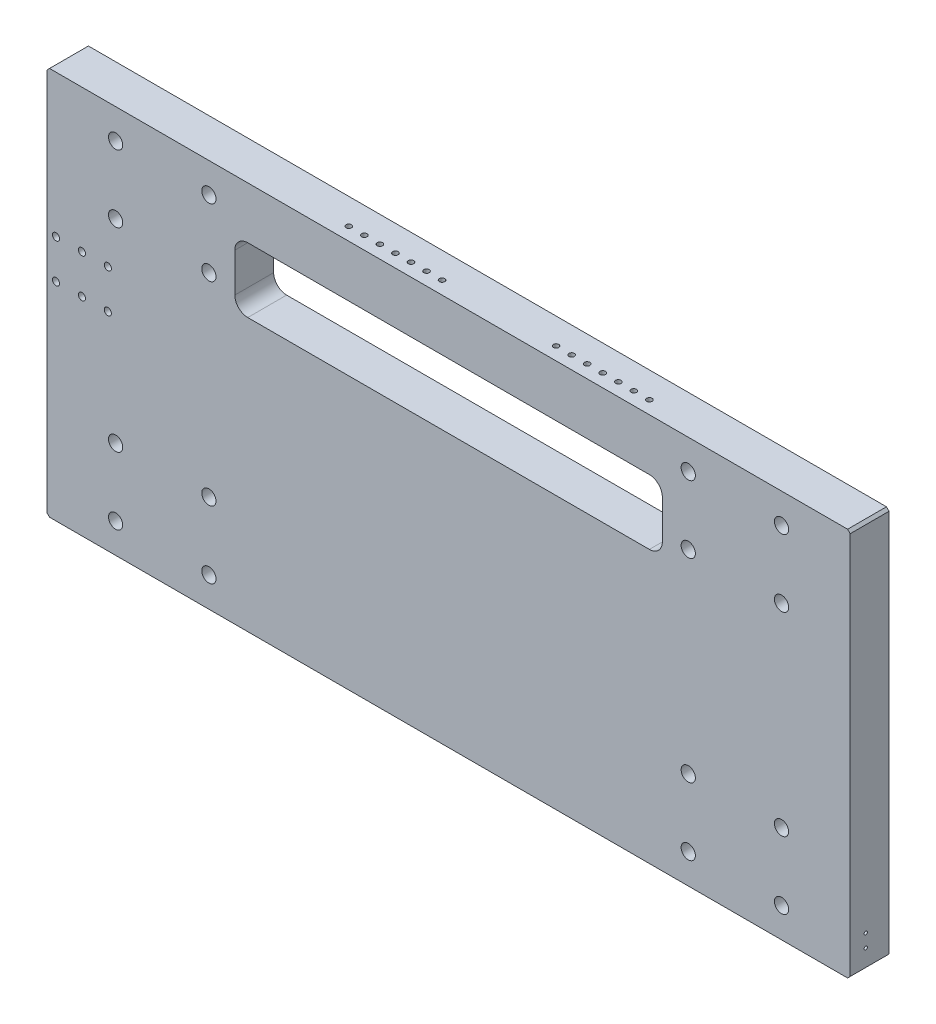
from build123d import *

# Parameters (mm, degrees)
SKETCH1_W                                            = 620
SKETCH1_H                                            = 300
BOSS_EXTRUDE1_DEPTH                                  = 15
CUT_EXTRUDE2_DEPTH                                   = 346.687720349
CHAMFER1_SIZE                                        = 2
M12_TAPPED_HOLE1_AT_2_COUNT                          = 2
M12_TAPPED_HOLE1_AT_2_PITCH                          = 190
M12_TAPPED_HOLE1_AT_3_COUNT                          = 2
M12_TAPPED_HOLE1_AT_3_PITCH                          = 447.353327919
M12_TAPPED_HOLE1_AT_4_COUNT                          = 2
M12_TAPPED_HOLE1_AT_4_PITCH                          = 405
LPATTERN1_COUNT                                      = 2
LPATTERN1_PITCH                                      = 35
M5_TAPPED_HOLE1_D                                    = 4.2
M5_TAPPED_HOLE1_DEPTH                                = 12.4
M5_TAPPED_HOLE1_TIP                                  = 1.2618073
F_4_0_4_DIAMETER_HOLE1_D                             = 4
F_4_0_4_DIAMETER_HOLE1_DEPTH                         = 12
F_4_0_4_DIAMETER_HOLE1_TIP                           = 1.201721238
HOLE_SIZE_PER_SOCKET_HEAD_CAP_SCREW_TYPE_D           = 11
HOLE_SIZE_PER_SOCKET_HEAD_CAP_SCREW_TYPE_CBORE_D     = 18
HOLE_SIZE_PER_SOCKET_HEAD_CAP_SCREW_TYPE_CBORE_DEPTH = 11
HOLE_SIZE_PER_SOCKET_HEAD_CAP_SCREW_2_D              = 5.5
HOLE_SIZE_PER_SOCKET_HEAD_CAP_SCREW_2_CBORE_D        = 10
HOLE_SIZE_PER_SOCKET_HEAD_CAP_SCREW_2_CBORE_DEPTH    = 5.7
M3_TAPPED_HOLE2_AT_2_COUNT                           = 2
M3_TAPPED_HOLE2_AT_2_PITCH                           = 10
M5_TAPPED_HOLE2_D                                    = 4.2
M5_TAPPED_HOLE2_DEPTH                                = 14
M5_TAPPED_HOLE2_TIP                                  = 1.2618073
M8_TAPPED_HOLE1_D                                    = 6.8
M8_TAPPED_HOLE1_DEPTH                                = 26.25
M8_TAPPED_HOLE1_TIP                                  = 2.042926105
M5_TAPPED_HOLE3_D                                    = 4.2
M5_TAPPED_HOLE3_DEPTH                                = 12.4
M5_TAPPED_HOLE3_TIP                                  = 1.2618073


with BuildPart() as part:
    # Sketch1 → Boss-Extrude1 (new, symmetric)
    with BuildSketch(Plane.XY):
        Rectangle(SKETCH1_W, SKETCH1_H)
    extrude(amount=BOSS_EXTRUDE1_DEPTH, both=True)

    # Sketch3 → Cut-Extrude2 (cut, through all)
    with BuildSketch(Plane(origin=(0, 0, -15), x_dir=(-1, 0, 0), z_dir=(0, 0, -1))):
        with BuildLine():
            Line((-155, 110), (155, 110))
            ThreePointArc((155, 110), (162.071067812, 107.071067812), (165, 100))
            Line((165, 100), (165, 70))
            ThreePointArc((165, 70), (162.071067812, 62.928932188), (155, 60))
            Line((155, 60), (-155, 60))
            ThreePointArc((-155, 60), (-162.071067812, 62.928932188), (-165, 70))
            Line((-165, 70), (-165, 100))
            ThreePointArc((-165, 100), (-162.071067812, 107.071067812), (-155, 110))
        make_face()
    extrude(amount=-CUT_EXTRUDE2_DEPTH, mode=Mode.SUBTRACT)

    # Chamfer1
    chamfer1_edges = [part.edges().sort_by_distance(p)[0] for p in [
        (310, -150, 0),
        (-310, -150, 0),
        (-310, 150, 0),
        (310, 150, 0),
    ]]
    chamfer(chamfer1_edges, length=CHAMFER1_SIZE)

    # Sketch9 → M12 Tapped Hole1 (revolve, cut)
    with BuildSketch(Plane(origin=(202.5, 125, -15), x_dir=(0, 1, 0), z_dir=(1, 0, 0))):
        Polygon((0, 0), (0, 28.314389157), (5.1, 25.25), (5.1, 0), align=None)
    m12_tapped_hole1 = revolve(axis=Axis((202.5, 125, -21.35), (0, 0, 1)), mode=Mode.SUBTRACT)

    # M12 Tapped Hole1 at 2: M12 Tapped Hole1 ×2
    with Locations(*[(0, -i * M12_TAPPED_HOLE1_AT_2_PITCH, 0) for i in range(1, M12_TAPPED_HOLE1_AT_2_COUNT)]):
        add(m12_tapped_hole1, mode=Mode.SUBTRACT)

    # M12 Tapped Hole1 at 3: M12 Tapped Hole1 ×2
    with Locations(*[Vector(-0.9053246611223111, -0.42472021139071386, 0) * (i * M12_TAPPED_HOLE1_AT_3_PITCH) for i in range(1, M12_TAPPED_HOLE1_AT_3_COUNT)]):
        add(m12_tapped_hole1, mode=Mode.SUBTRACT)

    # M12 Tapped Hole1 at 4: M12 Tapped Hole1 ×2
    with Locations(*[(-i * M12_TAPPED_HOLE1_AT_4_PITCH, 0, 0) for i in range(1, M12_TAPPED_HOLE1_AT_4_COUNT)]):
        add(m12_tapped_hole1, mode=Mode.SUBTRACT)

    # LPattern1: M12 Tapped Hole1 ×2
    with Locations(*[(-i * LPATTERN1_PITCH, 0, 0) for i in range(1, LPATTERN1_COUNT)]):
        add(m12_tapped_hole1, mode=Mode.SUBTRACT)

    # LPattern1 copy 1 sketch → LPattern1 copy 1 (revolve, cut)
    with BuildSketch(Plane(origin=(167.5, -65, -15), x_dir=(0, 1, 0), z_dir=(1, 0, 0))):
        Polygon((0, 0), (0, 28.314389157), (5.1, 25.25), (5.1, 0), align=None)
    revolve(axis=Axis((167.5, -65, -21.35), (0, 0, 1)), mode=Mode.SUBTRACT)

    # LPattern1 copy 2 sketch → LPattern1 copy 2 (revolve, cut)
    with BuildSketch(Plane(origin=(-237.5, -65, -15), x_dir=(0, 1, 0), z_dir=(1, 0, 0))):
        Polygon((0, 0), (0, 28.314389157), (5.1, 25.25), (5.1, 0), align=None)
    revolve(axis=Axis((-237.5, -65, -21.35), (0, 0, 1)), mode=Mode.SUBTRACT)

    # LPattern1 copy 3 sketch → LPattern1 copy 3 (revolve, cut)
    with BuildSketch(Plane(origin=(-237.5, 125, -15), x_dir=(0, 1, 0), z_dir=(1, 0, 0))):
        Polygon((0, 0), (0, 28.314389157), (5.1, 25.25), (5.1, 0), align=None)
    revolve(axis=Axis((-237.5, 125, -21.35), (0, 0, 1)), mode=Mode.SUBTRACT)

    # M5 Tapped Hole1
    with Locations(Plane(origin=(0, 0, -15), x_dir=(-1, 0, 0), z_dir=(0, 0, -1))):
        with Locations((-220, 45), (-110, 45), (0, 45), (110, 45), (220, 45), (220, -90), (110, -90), (0, -90), (-110, -90), (-220, -90)):
            Hole(M5_TAPPED_HOLE1_D / 2, depth=M5_TAPPED_HOLE1_DEPTH)
            with Locations((0, 0, -(M5_TAPPED_HOLE1_DEPTH + M5_TAPPED_HOLE1_TIP / 2))):  # 118° drill point
                Cone(0, M5_TAPPED_HOLE1_D / 2, M5_TAPPED_HOLE1_TIP, mode=Mode.SUBTRACT)

    # Ø4.0 (4) Diameter Hole1
    with Locations(Plane(origin=(0, 0, -15), x_dir=(-1, 0, 0), z_dir=(0, 0, -1))):
        with Locations((150, -90), (-150, -90), (-150, 45), (150, 45)):
            Hole(F_4_0_4_DIAMETER_HOLE1_D / 2, depth=F_4_0_4_DIAMETER_HOLE1_DEPTH)
            with Locations((0, 0, -(F_4_0_4_DIAMETER_HOLE1_DEPTH + F_4_0_4_DIAMETER_HOLE1_TIP / 2))):  # 118° drill point
                Cone(0, F_4_0_4_DIAMETER_HOLE1_D / 2, F_4_0_4_DIAMETER_HOLE1_TIP, mode=Mode.SUBTRACT)

    # Hole size per socket head cap screw type (through all)
    with Locations(Plane(origin=(0, 0, -15), x_dir=(-1, 0, 0), z_dir=(0, 0, -1))):
        with Locations((-257, 127), (-185, 127), (-257, 75), (-185, 75), (-185, -75), (-257, -75), (-257, -127), (-185, -127), (185, 127), (257, 127), (185, 75), (257, 75), (185, -75), (257, -75), (185, -127), (257, -127)):
            CounterBoreHole(HOLE_SIZE_PER_SOCKET_HEAD_CAP_SCREW_TYPE_D / 2, HOLE_SIZE_PER_SOCKET_HEAD_CAP_SCREW_TYPE_CBORE_D / 2, HOLE_SIZE_PER_SOCKET_HEAD_CAP_SCREW_TYPE_CBORE_DEPTH)

    # Hole size per socket head cap screw  2 (through all)
    with Locations(Plane(origin=(0, 0, -15), x_dir=(-1, 0, 0), z_dir=(0, 0, -1))):
        with Locations((263, 40), (303, 40), (303, 10), (263, 10), (283, 40), (283, 10)):
            CounterBoreHole(HOLE_SIZE_PER_SOCKET_HEAD_CAP_SCREW_2_D / 2, HOLE_SIZE_PER_SOCKET_HEAD_CAP_SCREW_2_CBORE_D / 2, HOLE_SIZE_PER_SOCKET_HEAD_CAP_SCREW_2_CBORE_DEPTH)

    # Sketch27 → M3 Tapped Hole2 (revolve, cut)
    with BuildSketch(Plane(origin=(-310, -135, 3), x_dir=(0, 0, 1), z_dir=(0, 1, 0))):
        Polygon((0, 0), (0, 8.251075774), (1.25, 7.5), (1.25, 0), align=None)
    m3_tapped_hole2 = revolve(axis=Axis((-316.35, -135, 3), (1, 0, 0)), mode=Mode.SUBTRACT)

    # M3 Tapped Hole2 at 2: M3 Tapped Hole2 ×2
    with Locations(*[(0, i * M3_TAPPED_HOLE2_AT_2_PITCH, 0) for i in range(1, M3_TAPPED_HOLE2_AT_2_COUNT)]):
        add(m3_tapped_hole2, mode=Mode.SUBTRACT)

    # Mirror2: M3 Tapped Hole2 across plane
    add(m3_tapped_hole2.mirror(Plane(origin=(0, 0, 0), x_dir=(0, 0, 1), z_dir=(1, 0, 0))), mode=Mode.SUBTRACT)

    # Mirror2 copy 1 sketch → Mirror2 copy 1 (revolve, cut)
    with BuildSketch(Plane(origin=(310, -125, 3), x_dir=(0, 0, 1), z_dir=(0, 1, 0))):
        Polygon((0, 0), (0, -8.251075774), (1.25, -7.5), (1.25, 0), align=None)
    revolve(axis=Axis((316.35, -125, 3), (1, 0, 0)), mode=Mode.SUBTRACT)

    # M5 Tapped Hole2
    with Locations(Plane(origin=(0, 0, -15), x_dir=(-1, 0, 0), z_dir=(0, 0, -1))):
        with Locations((263, 60), (263, 30), (263, 0), (303, 0), (303, 30), (303, 60)):
            Hole(M5_TAPPED_HOLE2_D / 2, depth=M5_TAPPED_HOLE2_DEPTH)
            with Locations((0, 0, -(M5_TAPPED_HOLE2_DEPTH + M5_TAPPED_HOLE2_TIP / 2))):  # 118° drill point
                Cone(0, M5_TAPPED_HOLE2_D / 2, M5_TAPPED_HOLE2_TIP, mode=Mode.SUBTRACT)

    # M8 Tapped Hole1
    with Locations(Plane(origin=(0, 0, -15), x_dir=(-1, 0, 0), z_dir=(0, 0, -1))):
        with Locations((-300, 0), (-300, -40)):
            Hole(M8_TAPPED_HOLE1_D / 2, depth=M8_TAPPED_HOLE1_DEPTH)
            with Locations((0, 0, -(M8_TAPPED_HOLE1_DEPTH + M8_TAPPED_HOLE1_TIP / 2))):  # 118° drill point
                Cone(0, M8_TAPPED_HOLE1_D / 2, M8_TAPPED_HOLE1_TIP, mode=Mode.SUBTRACT)

    # M5 Tapped Hole3
    with Locations(Plane(origin=(0, 150, 0), x_dir=(-1, 0, 0), z_dir=(0, 1, 0))):
        with Locations((-145, 5), (-133, 5), (-121, 5), (-109, 5), (-97, 5), (-85, 5), (15, 5), (27, 5), (39, 5), (51, 5), (63, 5), (75, 5), (-73, 5), (87, 5)):
            Hole(M5_TAPPED_HOLE3_D / 2, depth=M5_TAPPED_HOLE3_DEPTH)
            with Locations((0, 0, -(M5_TAPPED_HOLE3_DEPTH + M5_TAPPED_HOLE3_TIP / 2))):  # 118° drill point
                Cone(0, M5_TAPPED_HOLE3_D / 2, M5_TAPPED_HOLE3_TIP, mode=Mode.SUBTRACT)


solid = part.part
